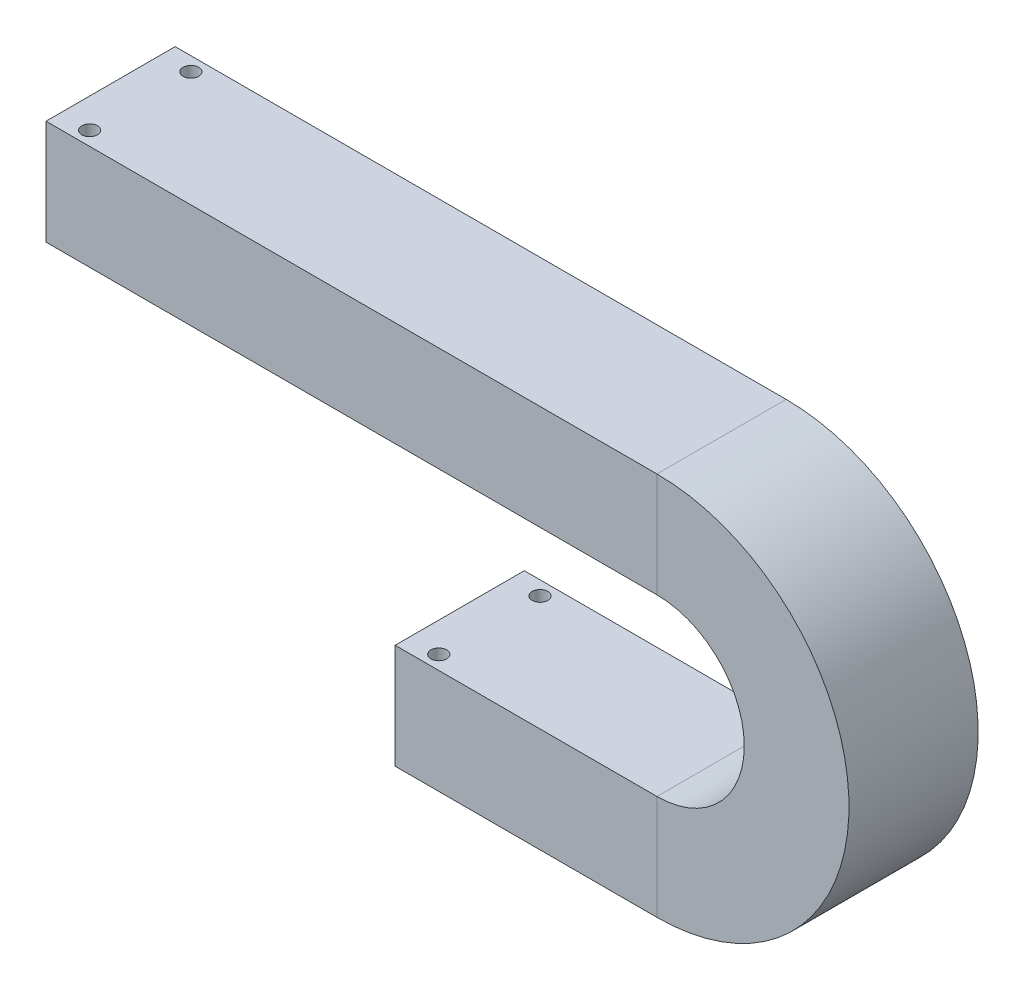
from build123d import *

# Parameters (mm, degrees)
SKETCH1_W                = 37
SKETCH1_H                = 30
SKETCH1_W_2              = 20
SKETCH1_H_2              = 20
M4_CLEARANCE_HOLE1_D     = 4.5
M4_CLEARANCE_HOLE1_DEPTH = 30
M4_CLEARANCE_HOLE2_D     = 4.5


with BuildPart() as part:
    # Sweep1: sweep along a path in Sketch2
    with BuildLine(Plane.XY) as sweep1_path:
        Line((0, 0), (75, 0))
        ThreePointArc((75, 0), (115, 40), (75, 80))
        Line((75, 80), (-100, 80))
    # Sketch1 → Sweep1 (sweep)
    with BuildSketch(Plane(origin=(0, 0, 0), x_dir=(0, 0, -1), z_dir=(1, 0, 0))):
        Rectangle(SKETCH1_W, SKETCH1_H)
        Rectangle(SKETCH1_W_2, SKETCH1_H_2, mode=Mode.SUBTRACT)
    sweep(path=sweep1_path.line)

    # M4 Clearance Hole1
    with Locations(Plane(origin=(0, 15, 0), x_dir=(1, 0, 0), z_dir=(0, 1, 0))):
        with Locations((8.5, 14.5), (8.5, -14.5)):
            Hole(M4_CLEARANCE_HOLE1_D / 2, depth=M4_CLEARANCE_HOLE1_DEPTH)

    # M4 Clearance Hole2 (through all)
    with Locations(Plane(origin=(0, 95, 0), x_dir=(1, 0, 0), z_dir=(0, 1, 0))):
        with Locations((-91.5, -14.5), (-91.5, 14.5)):
            Hole(M4_CLEARANCE_HOLE2_D / 2)


solid = part.part
